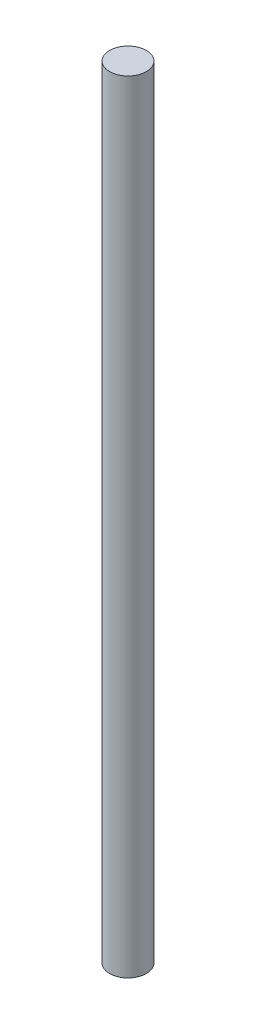
SolidWorks part; units mm, degrees
ref_plane "Front Plane" through (0, 0, 0) normal (0, 0, 1) x (1, 0, 0)
ref_plane "Top Plane" through (0, 0, 0) normal (0, 1, 0) x (1, 0, 0)
ref_plane "Right Plane" through (0, 0, 0) normal (1, 0, 0) x (0, 0, -1)
sketch "Sketch1" plane through (0, 0, 0) normal (0, 1, 0) x (1, 0, 0)
  circle A0 centre (0, 0) radius 2
extrude "Boss-Extrude1" add sketch "Sketch1" along normal blind 85
